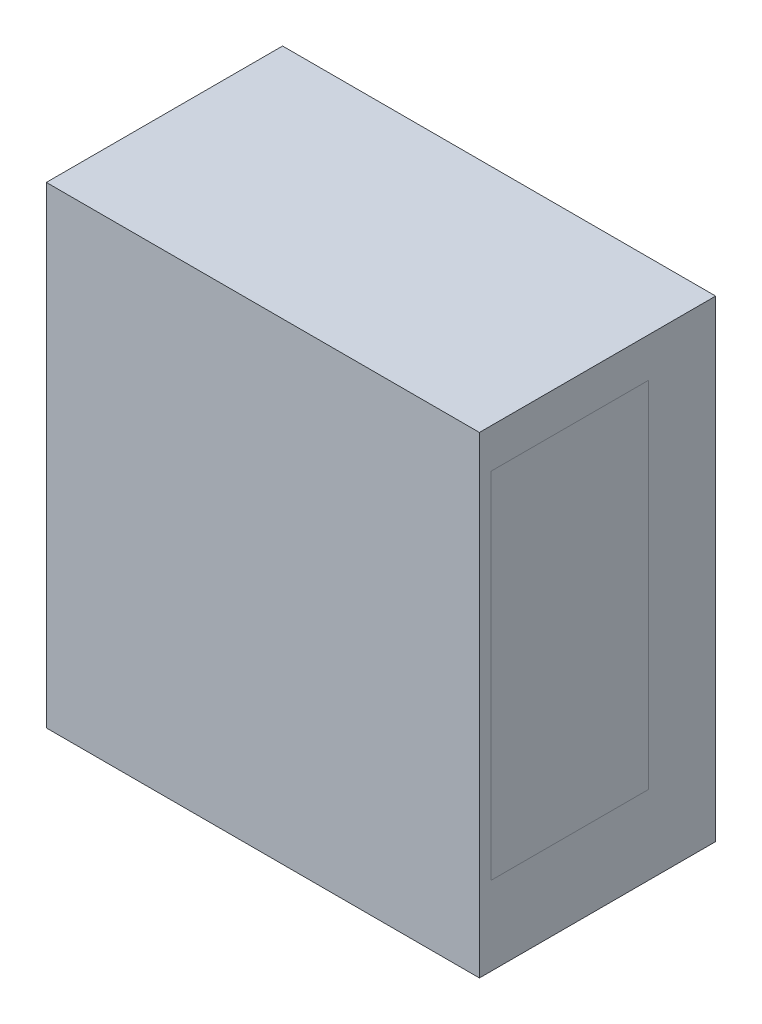
from build123d import *

# Parameters (mm, degrees)
SKETCH_1_W             = 110
SKETCH_1_H             = 120
EXTRUDE_1_DEPTH        = 30
HOLE_WIZARD_M4_1_D     = 3.3
HOLE_WIZARD_M4_1_DEPTH = 10.1
HOLE_WIZARD_M4_1_TIP   = 0.991420021


with BuildPart() as part:
    # 草图1 → 凸台-拉伸1 (new, symmetric)
    with BuildSketch(Plane.XY):
        Rectangle(SKETCH_1_W, SKETCH_1_H)
    extrude(amount=EXTRUDE_1_DEPTH, both=True)

    # M4 螺纹孔1
    with Locations(Plane(origin=(0, 0, -30), x_dir=(-1, 0, 0), z_dir=(0, 0, -1))):
        with Locations((0, 15), (0, -15)):
            Hole(HOLE_WIZARD_M4_1_D / 2, depth=HOLE_WIZARD_M4_1_DEPTH)
            with Locations((0, 0, -(HOLE_WIZARD_M4_1_DEPTH + HOLE_WIZARD_M4_1_TIP / 2))):  # 118° drill point
                Cone(0, HOLE_WIZARD_M4_1_D / 2, HOLE_WIZARD_M4_1_TIP, mode=Mode.SUBTRACT)


solid = part.part
